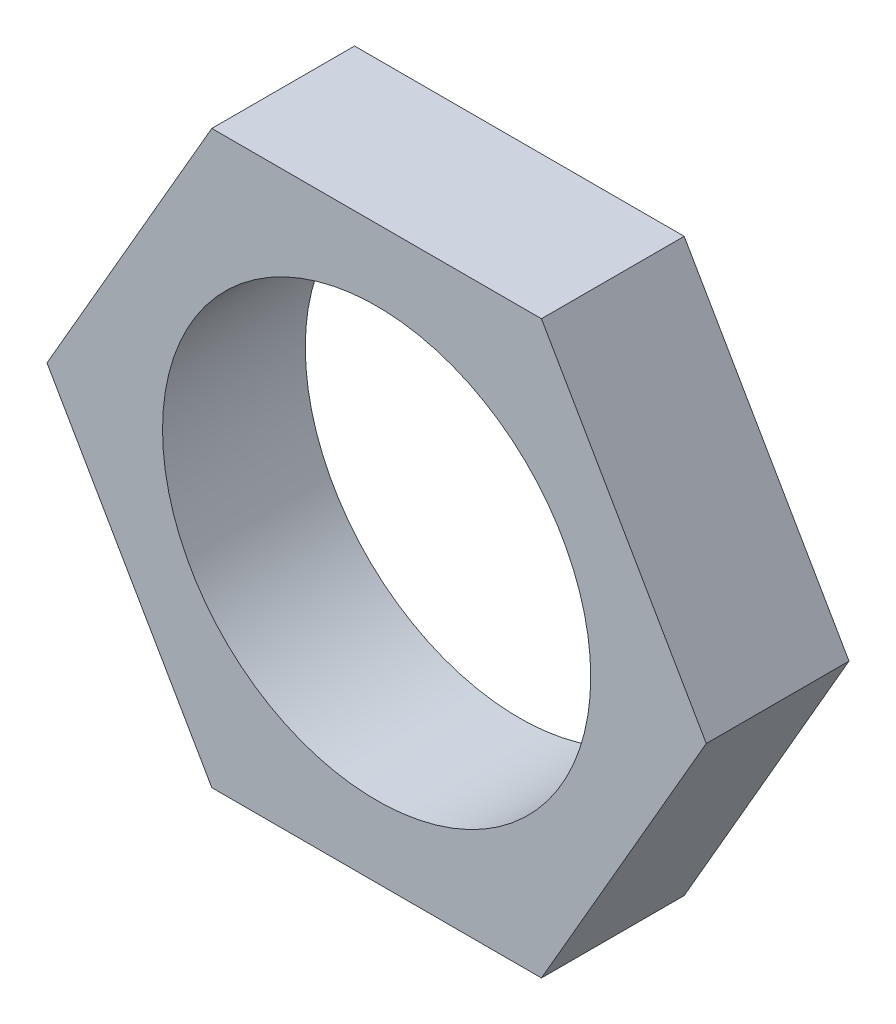
from build123d import *

# Parameters (mm, degrees)
BOSS_EXTRUDE1_DEPTH        = 3
M10X1_0_TAPPED_HOLE1_D     = 9
M10X1_0_TAPPED_HOLE1_DEPTH = 23
M10X1_0_TAPPED_HOLE1_TIP   = 2.703872786


with BuildPart() as part:
    # Sketch1 → Boss-Extrude1 (new body)
    with BuildSketch(Plane.XY):
        Polygon((6.92820323, 0), (3.464101615, 6), (-3.464101615, 6), (-6.92820323, 0), (-3.464101615, -6), (3.464101615, -6), align=None)
    extrude(amount=BOSS_EXTRUDE1_DEPTH)

    # M10x1.0 Tapped Hole1
    with Locations(Plane.XY.offset(3)):
        with Locations((0, 0)):
            Hole(M10X1_0_TAPPED_HOLE1_D / 2, depth=M10X1_0_TAPPED_HOLE1_DEPTH)
            with Locations((0, 0, -(M10X1_0_TAPPED_HOLE1_DEPTH + M10X1_0_TAPPED_HOLE1_TIP / 2))):  # 118° drill point
                Cone(0, M10X1_0_TAPPED_HOLE1_D / 2, M10X1_0_TAPPED_HOLE1_TIP, mode=Mode.SUBTRACT)


solid = part.part
